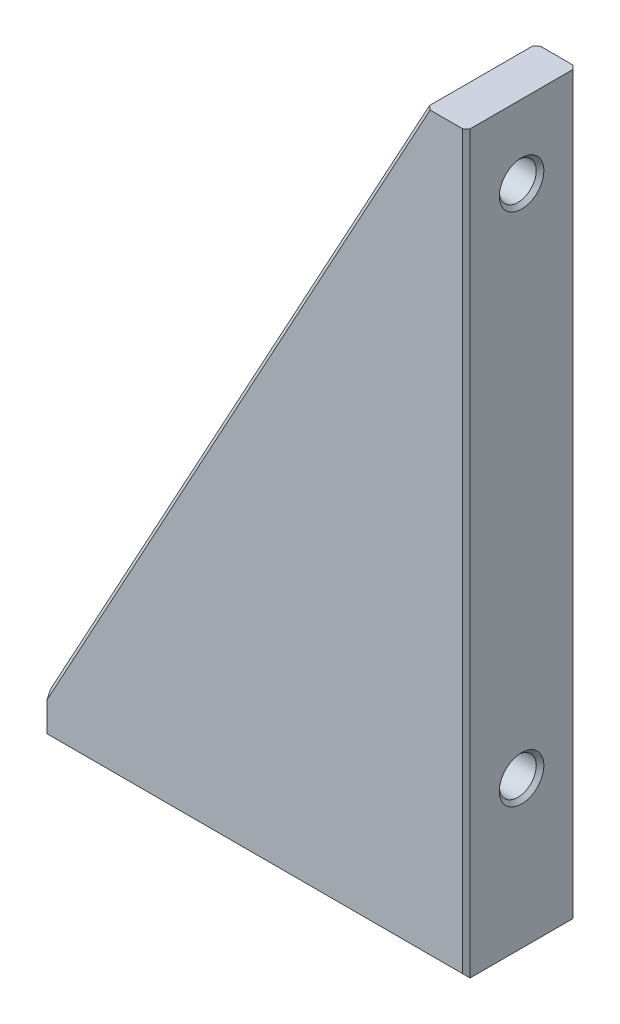
SolidWorks part; units mm, degrees
material "45#"
ref_plane "前视基准面" through (0, 0, 0) normal (0, 0, 1) x (1, 0, 0)
ref_plane "上视基准面" through (0, 0, 0) normal (0, 1, 0) x (1, 0, 0)
ref_plane "右视基准面" through (0, 0, 0) normal (1, 0, 0) x (0, 0, -1)
sketch "草图1" plane through (0, 0, 0) normal (0, 0, 1) x (1, 0, 0)
  line L0 (0, 0) -> (60, 0)
  line L1 (60, 0) -> (60, 110)
  line L2 (60, 110) -> (0, 0)
  dimension "D1" = 60
  dimension "D2" = 110
extrude "凸台-拉伸1" add sketch "草图1" along normal blind 15
hole_wizard "M6 螺纹孔1" positions "草图2" profile "草图3" tap size "M6" standard "AS"
sketch "草图2" plane through (0, 0, 0) normal (0, -1, 0) x (-1, 0, 0)
  line L0 (0, 0) -> (-60, 0) construction
  line L1 (-60, -15) -> (-60, 0) construction
  line L2 (0, -15) -> (0, 0) construction
  point P0 (-48, -7.5)
  point P6 (-12, -7.5)
  dimension "D1" = 7.5
  dimension "D2" = 12
  dimension "D3" = 12
sketch "草图3" plane through (48, 0, 7.5) normal (1, 0, 0) x (0, 0, -1)
  line L0 (0, 0) -> (0, 16.5022)
  line L1 (0, 16.5022) -> (2.5, 15)
  line L2 (2.5, 15) -> (2.5, 0.7243)
  line L3 (2.5, 0.7243) -> (3.25, 0)
  line L5 (3.25, 0) -> (0, 0)
  line L6 (-2.5, 0.7243) -> (-3.25, 0) construction
  line L10 (0, 16.5022) -> (-2.5, 15) construction
  line L11 (0, -6.35) -> (0, 107.95) construction
  dimension "螺纹孔钻头直径" = 5
  dimension "螺纹孔钻头深度" = 15
  dimension "近端锥形沉头孔直径" = 6.5
  dimension "近端锥形沉头孔角度" = 92
  dimension "导头角度" = 118
cosmetic thread "孔螺蚊线1" parameters "D1"=12, "D2"=6
cosmetic thread "孔螺蚊线2" parameters "D1"=12, "D2"=6
hole_wizard "M6 螺纹孔2" positions "草图4" profile "草图6" tap size "M6" standard "AS"
sketch "草图4" plane through (60, 0, 0) normal (1, 0, 0) x (0, 0, -1)
  line L0 (-15, 0) -> (-15, 110) construction
  line L1 (-15, 0) -> (0, 0) construction
  line L2 (-15, 110) -> (0, 110) construction
  point P0 (-7.5, 20)
  point P3 (-7.5, 90)
  dimension "D1" = 7.5
  dimension "D2" = 7.5
  dimension "D3" = 20
  dimension "D4" = 20
sketch "草图6" plane through (60, 20, 7.5) normal (0, 1, 0) x (0, 0, -1)
  line L0 (0, 0) -> (0, 16.5022)
  line L1 (0, 16.5022) -> (2.5, 15)
  line L2 (2.5, 15) -> (2.5, 0.507)
  line L3 (2.5, 0.507) -> (3.025, 0)
  line L5 (3.025, 0) -> (0, 0)
  line L6 (-2.5, 0.507) -> (-3.025, 0) construction
  line L10 (0, 16.5022) -> (-2.5, 15) construction
  line L11 (0, -6.35) -> (0, 107.95) construction
  dimension "螺纹孔钻头直径" = 5
  dimension "螺纹孔钻头深度" = 15
  dimension "近端锥形沉头孔直径" = 6.05
  dimension "近端锥形沉头孔角度" = 92
  dimension "导头角度" = 118
cosmetic thread "孔螺蚊线3" parameters "D1"=12, "D2"=6
cosmetic thread "孔螺蚊线4" parameters "D1"=12, "D2"=6
chamfer "倒角1" distance 0.5 angle 45 6 edges at (60, 55, 0) (30, 55, 0) (30, 0, 0) (60, 55, 15) (30, 0, 15) (30, 55, 15)
sketch "草图7" plane through (0, 0, 15) normal (0, 0, 1) x (1, 0, 0)
  line L0 (0, 0) -> (60, 110) construction
  line L1 (60, 110) -> (54.5, 110)
  line L2 (60, 110) -> (60, 99.9167)
  line L3 (60, 99.9167) -> (54.5, 99.9167)
  line L4 (54.5, 110) -> (54.5, 99.9167)
  line L5 (0, 0) -> (3, 0)
  line L6 (0, 0) -> (0, 20)
  line L7 (0, 20) -> (3, 20)
  line L8 (3, 0) -> (3, 20)
  dimension "D1" = 5.5
  dimension "D3" = 3
  dimension "D4" = 20
extrude "切除-拉伸1" cut sketch "草图7" against normal through all
